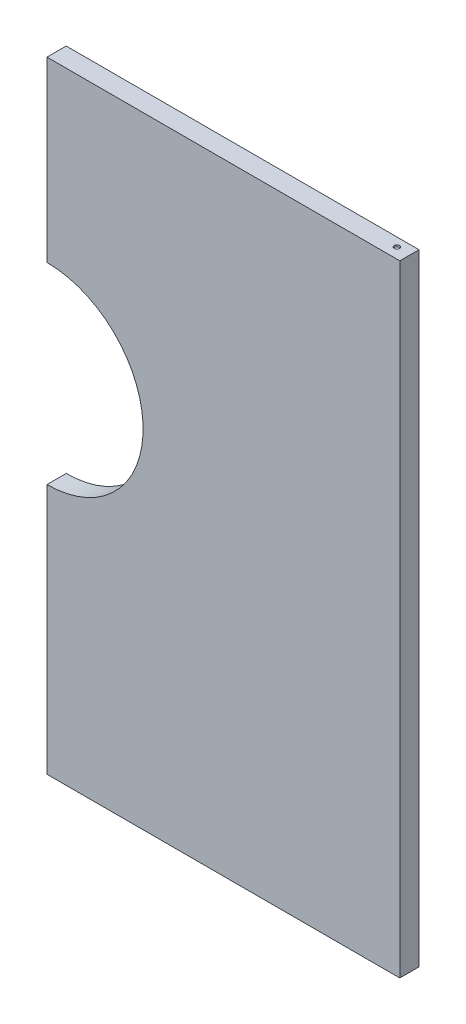
from build123d import *

# Parameters (mm, degrees)
EXTRUDE_1_DEPTH          = 20
SHELL_1_T                = -2
CUT_EXTRUDE_1_DEPTH      = 792
CUT_EXTRUDE_1_DEPTH_BACK = 76
SKETCH_2_R               = 2.75
SKETCH_3_R               = 2.75
CUT_EXTRUDE_2_DEPTH      = 10


with BuildPart() as part:
    # 草图1 → 凸台-拉伸1 (new body)
    with BuildSketch(Plane.XY):
        with BuildLine():
            Line((0, 461), (0, 646))
            Line((0, 646), (367, 646))
            Line((367, 646), (367, 0))
            Line((367, 0), (0, 0))
            Line((0, 0), (0, 261))
            ThreePointArc((0, 261), (100, 361), (0, 461))
        make_face()
    extrude(amount=EXTRUDE_1_DEPTH)

    # 抽壳1
    shell_1_openings = [part.faces().sort_by_distance(p)[0] for p in [
        (193.509053572, 320.303646747, 0),
    ]]
    offset(amount=SHELL_1_T, openings=shell_1_openings, kind=Kind.INTERSECTION)

    # 草图2 → 切除-拉伸1 (cut, two sides: drawn at the far end of the back side and taken through both)
    with BuildSketch(Plane(origin=(0, 2, 0), x_dir=(1, 0, 0), z_dir=(0, 1, 0)).offset(-CUT_EXTRUDE_1_DEPTH_BACK)):
        with Locations(Location((353, -9, 0), (0, 0, 90))):
            Circle(SKETCH_2_R)
    extrude(amount=CUT_EXTRUDE_1_DEPTH + CUT_EXTRUDE_1_DEPTH_BACK, mode=Mode.SUBTRACT)

    # 草图3 → 切除-拉伸2 (cut)
    with BuildSketch(Plane(origin=(2, 0, 0), x_dir=(0, 0, -1), z_dir=(1, 0, 0))):
        with Locations((-9, 632)):
            Circle(SKETCH_3_R)
        with Locations((-9, 552)):
            Circle(SKETCH_3_R)
        with Locations((-9, 472)):
            Circle(SKETCH_3_R)
        with Locations((-9, 14)):
            Circle(SKETCH_3_R)
        with Locations((-9, 129)):
            Circle(SKETCH_3_R)
        with Locations((-9, 244)):
            Circle(SKETCH_3_R)
    extrude(amount=-CUT_EXTRUDE_2_DEPTH, mode=Mode.SUBTRACT)


solid = part.part
